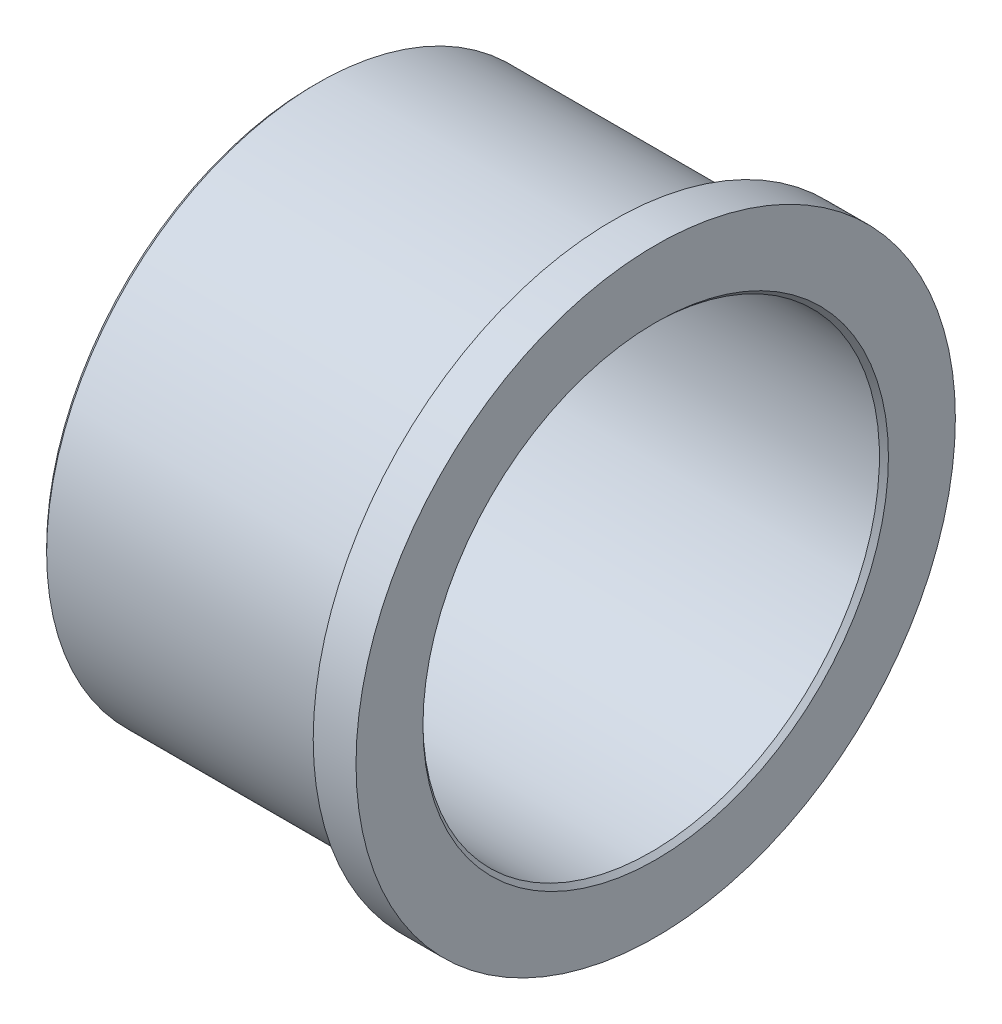
from build123d import *


with BuildPart() as part:
    # Sketch 181 → 旋转1 (revolve)
    with BuildSketch(Plane.XY, mode=Mode.PRIVATE) as revolve_1_sk:
        Polygon((-30, 40.77255102), (-29.2, 40), (29.2, 40), (30, 40.77255102), (30, 52.5), (22.5, 52.5), (22.5, 47.3), (20.5, 47.3), (20.5, 47.5), (-29.2, 47.5), (-30, 46.7), align=None)
    revolve(revolve_1_sk.sketch.rotate(Axis((-30, 0, 0), (1, 0, 0)), 90), axis=Axis((-30, 0, 0), (1, 0, 0)))


solid = part.part
